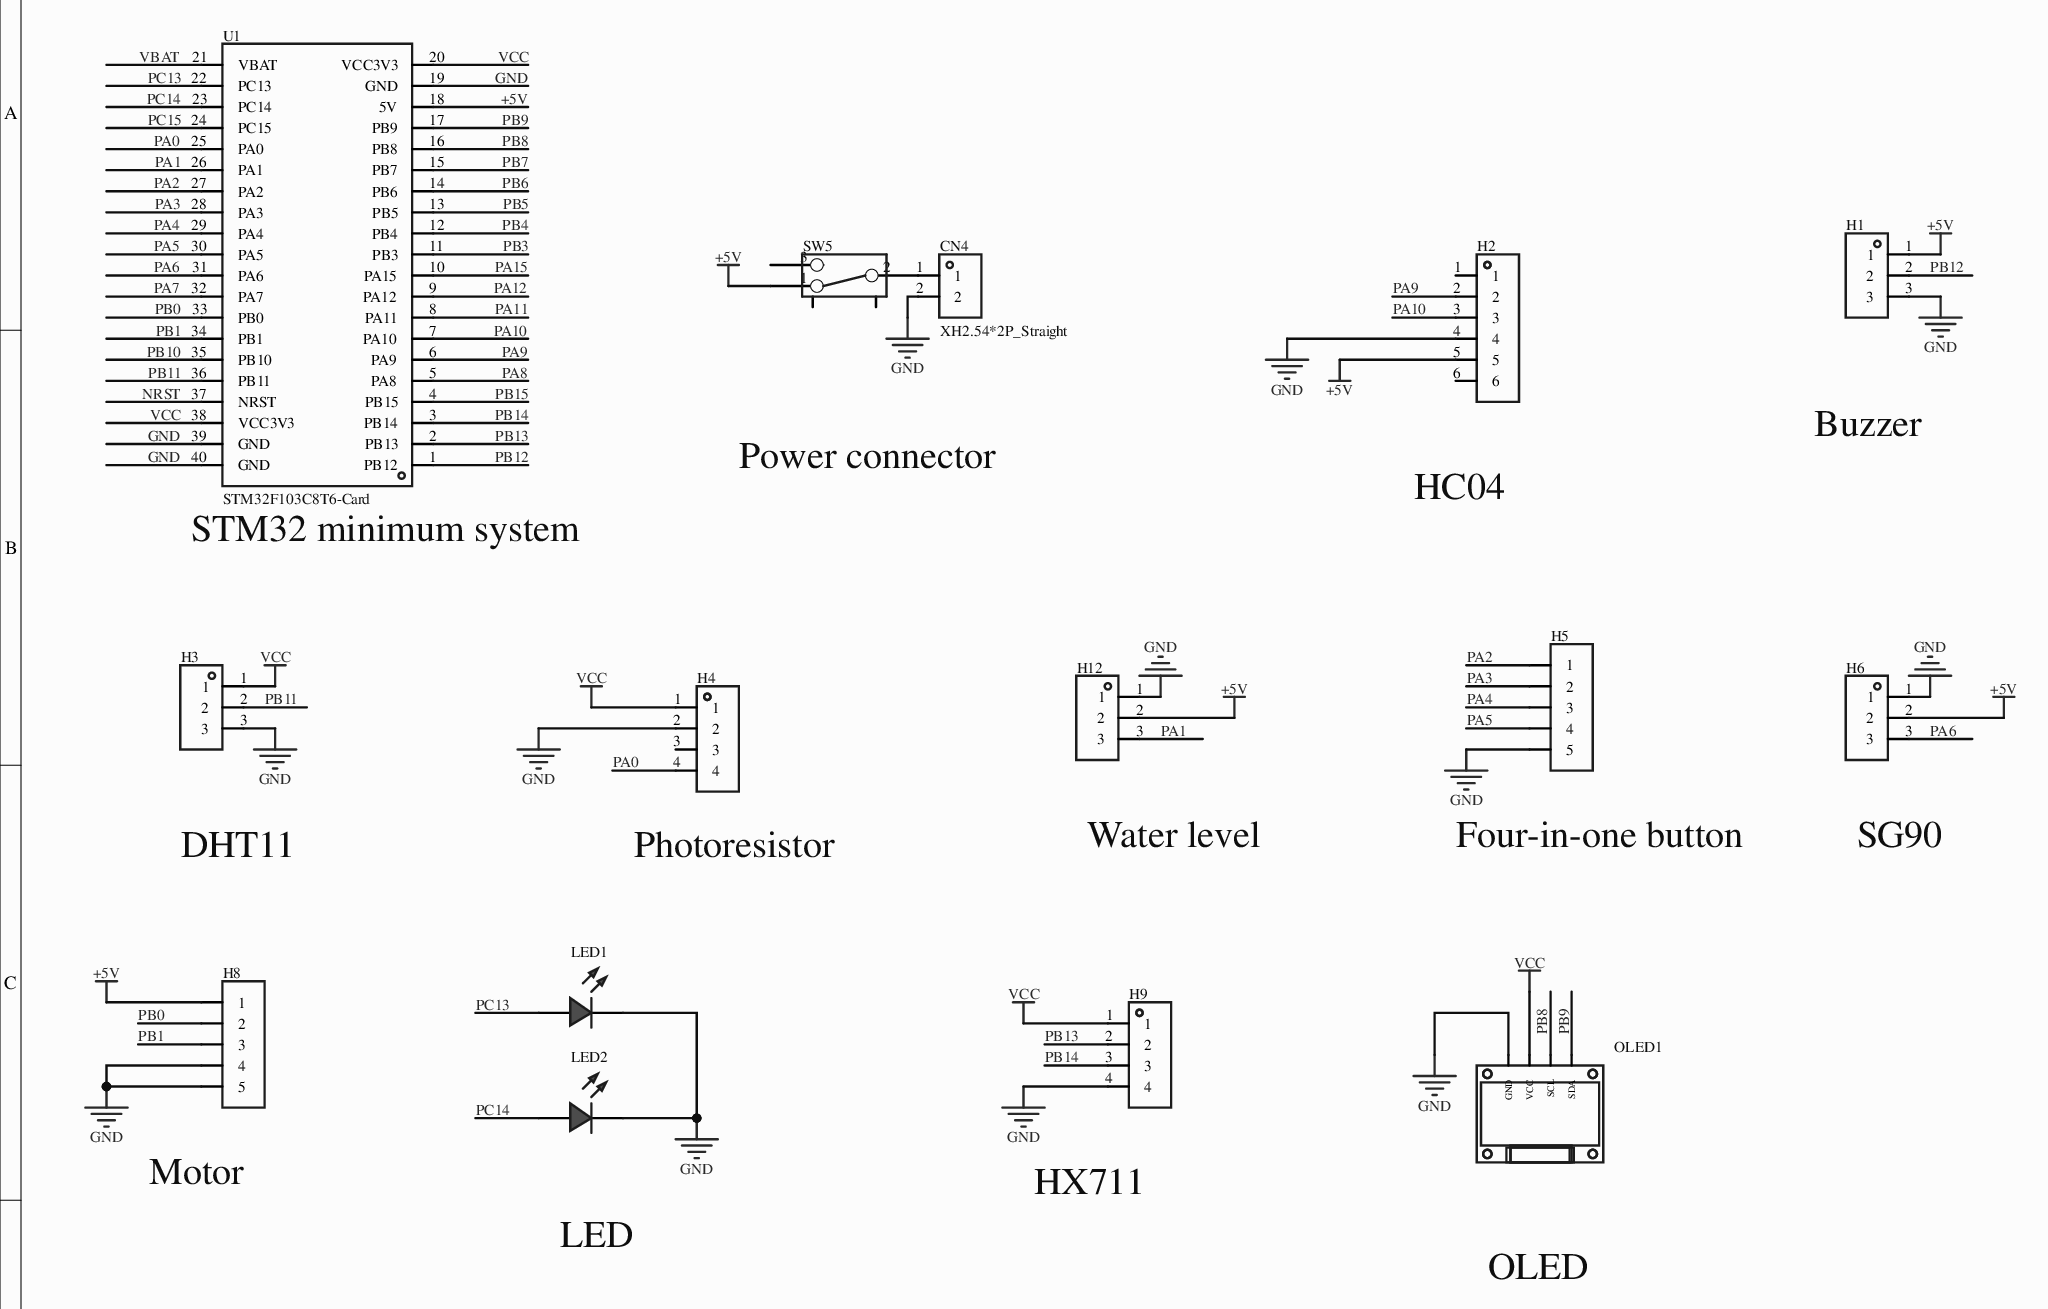
[diagram p0: MISC51952-3.schdoc]
# Altium project MISC51952-2.PrjPcb
1 sheet, 15 parts. Net scope: global (net labels, ports and power ports of the same name join across sheets).
Board file: MISC51952.pcbdoc

## Sheet MISC51952-3.schdoc
size 297 x 209 mm; Version: V1.0; @Project Name: MISC51952; @Page Count: 1; @Update Date: 2026-04-23; @Create Date: 2026-04-23; @Schematic Name: MISC51952; @Page No: 1; @Create Time: 23:22:16; @Update Time: 17:32:40; @Board Name: MISC51952

### Parts
CN4  XH2.54*2P_Straight  [CONN-TH_2P-P2.50-XH2.54-2P]
H1  (no value)  [HDR-TH_3P-P2.54-V-F]
H2  (no value)  [HDR-TH_6P-P2.54-V-F]
H3  (no value)  [HDR-TH_3P-P2.54-V-F]
H4  (no value)  [HDR-TH_4P-P2.54-V-F]
H5  (no value)  [HDR-TH_5P-P2.54-V-F]
H6  (no value)  [HDR-TH_3P-P2.54-V-F]
H8  (no value)  [HDR-TH_5P-P2.54-V-F]
H9  (no value)  [HDR-TH_4P-P2.54-V-F]
H12  (no value)  [HDR-TH_3P-P2.54-V-F]
LED1  (no value)  [LED-TH_5mm]
LED2  (no value)  [LED-TH_5mm]
OLED1  (no value)  [0.96OLED_4P]
SW5  (no value)  [拨动开关]
U1  STM32F103C8T6-Card  [CONN-TH_L53.3-W22.9_STM32F103C8T6-CARD]

### Nets
+5V: H1.1 H2.5 H6.2 H8.1 H12.2 SW5.1 U1.18(5V)
GND: CN4.2 H1.3 H2.4 H3.3 H4.2 H5.5 H6.1 H8.4 H8.5 H9.4 H12.1 LED1.2(A) LED2.2(A) OLED1.1(GND) U1.19(GND) U1.39(GND) U1.40(GND)
VCC: H3.1 H4.1 H9.1 OLED1.2(VCC) U1.20(VCC3V3) U1.38(VCC3V3)
NRST: U1.37(NRST)
PA0: H4.4 U1.25(PA0)
PA1: H12.3 U1.26(PA1)
PA2: H5.1 U1.27(PA2)
PA3: H5.2 U1.28(PA3)
PA4: H5.3 U1.29(PA4)
PA5: H5.4 U1.30(PA5)
PA6: H6.3 U1.31(PA6)
PA7: U1.32(PA7)
PA8: U1.5(PA8)
PA9: H2.2 U1.6(PA9)
PA10: H2.3 U1.7(PA10)
PA11: U1.8(PA11)
PA12: U1.9(PA12)
PA15: U1.10(PA15)
PB0: H8.2 U1.33(PB0)
PB1: H8.3 U1.34(PB1)
PB3: U1.11(PB3)
PB4: U1.12(PB4)
PB5: U1.13(PB5)
PB6: U1.14(PB6)
PB7: U1.15(PB7)
PB8: OLED1.3(SCL) U1.16(PB8)
PB9: OLED1.4(SDA) U1.17(PB9)
PB10: U1.35(PB10)
PB11: H3.2 U1.36(PB11)
PB12: H1.2 U1.1(PB12)
PB13: H9.2 U1.2(PB13)
PB14: H9.3 U1.3(PB14)
PB15: U1.4(PB15)
PC13: LED1.1(C) U1.22(PC13)
PC14: LED2.1(C) U1.23(PC14)
PC15: U1.24(PC15)
VBAT: U1.21(VBAT)
NetCN4_1: CN4.1 SW5.2

Not connected (* = marked no-connect by the designer): H2 1 6; H4 3; SW5 3 4 5

### Notes on the sheet
- Power connector
- HC04
- Buzzer
- (near U1) STM32 minimum system
- DHT11
- (near H4) Photoresistor
- (near H12) Water level
- (near H5) Four-in-one button
- (near H6) SG90
- (near H8) Motor
- LED
- (near H9) HX711
- OLED

### Library data of the parts
CN4 = XH2.54*2P_直插: 3D Model: 325c595e30db4df8abe76612dd40b0fa0819f05c4eef4c71ace90d822a990e87; 3D Model Transform: 295.275,228.346,0,180,0,0,-0.002,-20.079,-137.795; AddInBom: yes; Device: XH2.54*2P_Straight; Symbol: XH2.54*2P_Straight; LCSC Part Name: XH2.54*2P_直插; Supplier Part: C9900008615; Manufacturer Part: XH2.54*2P_直插; Supplier Footprint: XH2.54_2P; JLCPCB Part Class: Extended Part; Supplier: LCSC; FootprintName: CONN-TH_2P-P2.50-XH2.54-2P; ConvertToPcb: yes; ModelName: CONN-TH_2P-P2.50-XH2.54-2P
H1 H3 H6 H12 = HDR-F_2.54_1x3P: Symbol: PM254V-11-03-H85; 3D Model: f3b3cc5aae9641bf9e56fc160cef875b; 3D Model Transform: 299.9994,100,0,0,0,0,0,0,-118.11; ConvertToPcb: yes; ModelName: HDR2.54-F-LI-1X3P; Device: HDR-F_2.54_1x3P; Supplier Part: C541850; Supplier Footprint: 插件; FootprintName: HDR-TH_3P-P2.54-V-F; AddInBom: yes
H2 = HDR-F_2.54_1x6P: Symbol: Header-Female-2.54_1x6; ConvertToPcb: yes; ModelId: 0f5bcf94dcda47d085f24cdca1696fe9; ModelTransform: 619.684,94.488,0,0,0,0,0,0,-125.984; Device: HDR-F_2.54_1x6P; AddInBom: yes; SupplierPart: C40877; Supplier Footprint: 插件; FootprintName: HDR-TH_6P-P2.54-V-F; ModelName: HDR-TH_6P-P2.54-V-F
H4 = HDR-F_2.54_1x4P: Symbol: 2.54-1*4P female; ConvertToPcb: yes; ModelId: d187812051054f85879fcaa51a310d8e0819f05c4eef4c71ace90d822a990e87; ModelTransform: 419.6842,98.464,0,0,0,0,0,0,-118.11; Device: HDR-F_2.54_1x4P; FootprintName: HDR-TH_4P-P2.54-V-F; AddInBom: yes; SupplierPart: C2718488; Supplier Footprint: 插件; ModelName: HDR-TH_4P-P2.54-V-F
H5 H8 = HDR-F_2.54_1x5P: Symbol: Header-Female-2.54_1x5; ConvertToPcb: yes; ModelId: f49cb6116a3d45e5a64915bf3e00773f; ModelTransform: 519.684,98.464,0,0,0,0,0,0,-124.016; Device: HDR-F_2.54_1x5P; AddInBom: yes; SupplierPart: C50950; Supplier Footprint: 插件; FootprintName: HDR-TH_5P-P2.54-V-F; ModelName: HDR-TH_5P-P2.54-V-F
H9 = HDR-F_2.54_1x4P: Symbol: 2.54-1*4P female; 3D Model: d187812051054f85879fcaa51a310d8e0819f05c4eef4c71ace90d822a990e87; 3D Model Transform: 419.6842,98.464,0,0,0,0,0,0,-118.11; ConvertToPcb: yes; Device: HDR-F_2.54_1x4P; Supplier Part: C2718488; Supplier Footprint: 插件; FootprintName: HDR-TH_4P-P2.54-V-F; AddInBom: yes; ModelName: HDR-TH_4P-P2.54-V-F
LED1 LED2 = LED_TH-R_5mm: 3D Model: fe9cea1bdf7642cd8d9a5077ed0e2b580819f05c4eef4c71ace90d822a990e87; 3D Model Transform: 222.16,238.98,581.81,180,0,0,-6,0,-220; ConvertToPcb: yes; ModelName: LED-TH_BD5.9-P2.54-RD_RED; Symbol: LED_TH-R; Device: LED_TH-R_5mm; Supplier Footprint: 插件; AddInBom: yes; FootprintName: LED-TH_5mm
OLED1 = 0.96OLED模块_4P: Device: 0.96OLED module_4P; ConvertToPcb: yes; ModelId: 79c000fdb68d45a296c2e9bedf4f9055; ModelTransform: 1393.69792,1318.895,0,0,0,0,0,-560.079,-137.795; Symbol: 0.96OLED module_4P; FootprintName: 0.96OLED_4P; AddInBom: yes; Supplier Footprint: 插件; ModelName: 0.96OLED_4P
SW5 = 拨动开关_正: Device: Toggle switch_Pos; Symbol: Toggle switch; ConvertToPcb: yes; ModelId: 4321fe59a4074cbfb4989553f297c68f0819f05c4eef4c71ace90d822a990e87; ModelName: SW-TH_SS-12D02-VG4; ModelTransform: 370.09,208.7,472.35,0,0,0,0,0,-110; FootprintName: Toggle switch; AddInBom: yes; Supplier Footprint: 插件
U1 = STM32F103C8T6-Card: AddInBom: yes; Device: STM32F103C8T6-Card; Symbol: STM32F103C8T6-CARD; FootprintName: CONN-TH_L53.3-W22.9_STM32F103C8T6-CARD; LCSC Part Name: STM32F103C8T6-Card; SupplierPart: C9900077949; ManufacturerPart: STM32F103C8T6-Card; Supplier Footprint: 插件; Supplier: LCSC; ConvertToPcb: yes